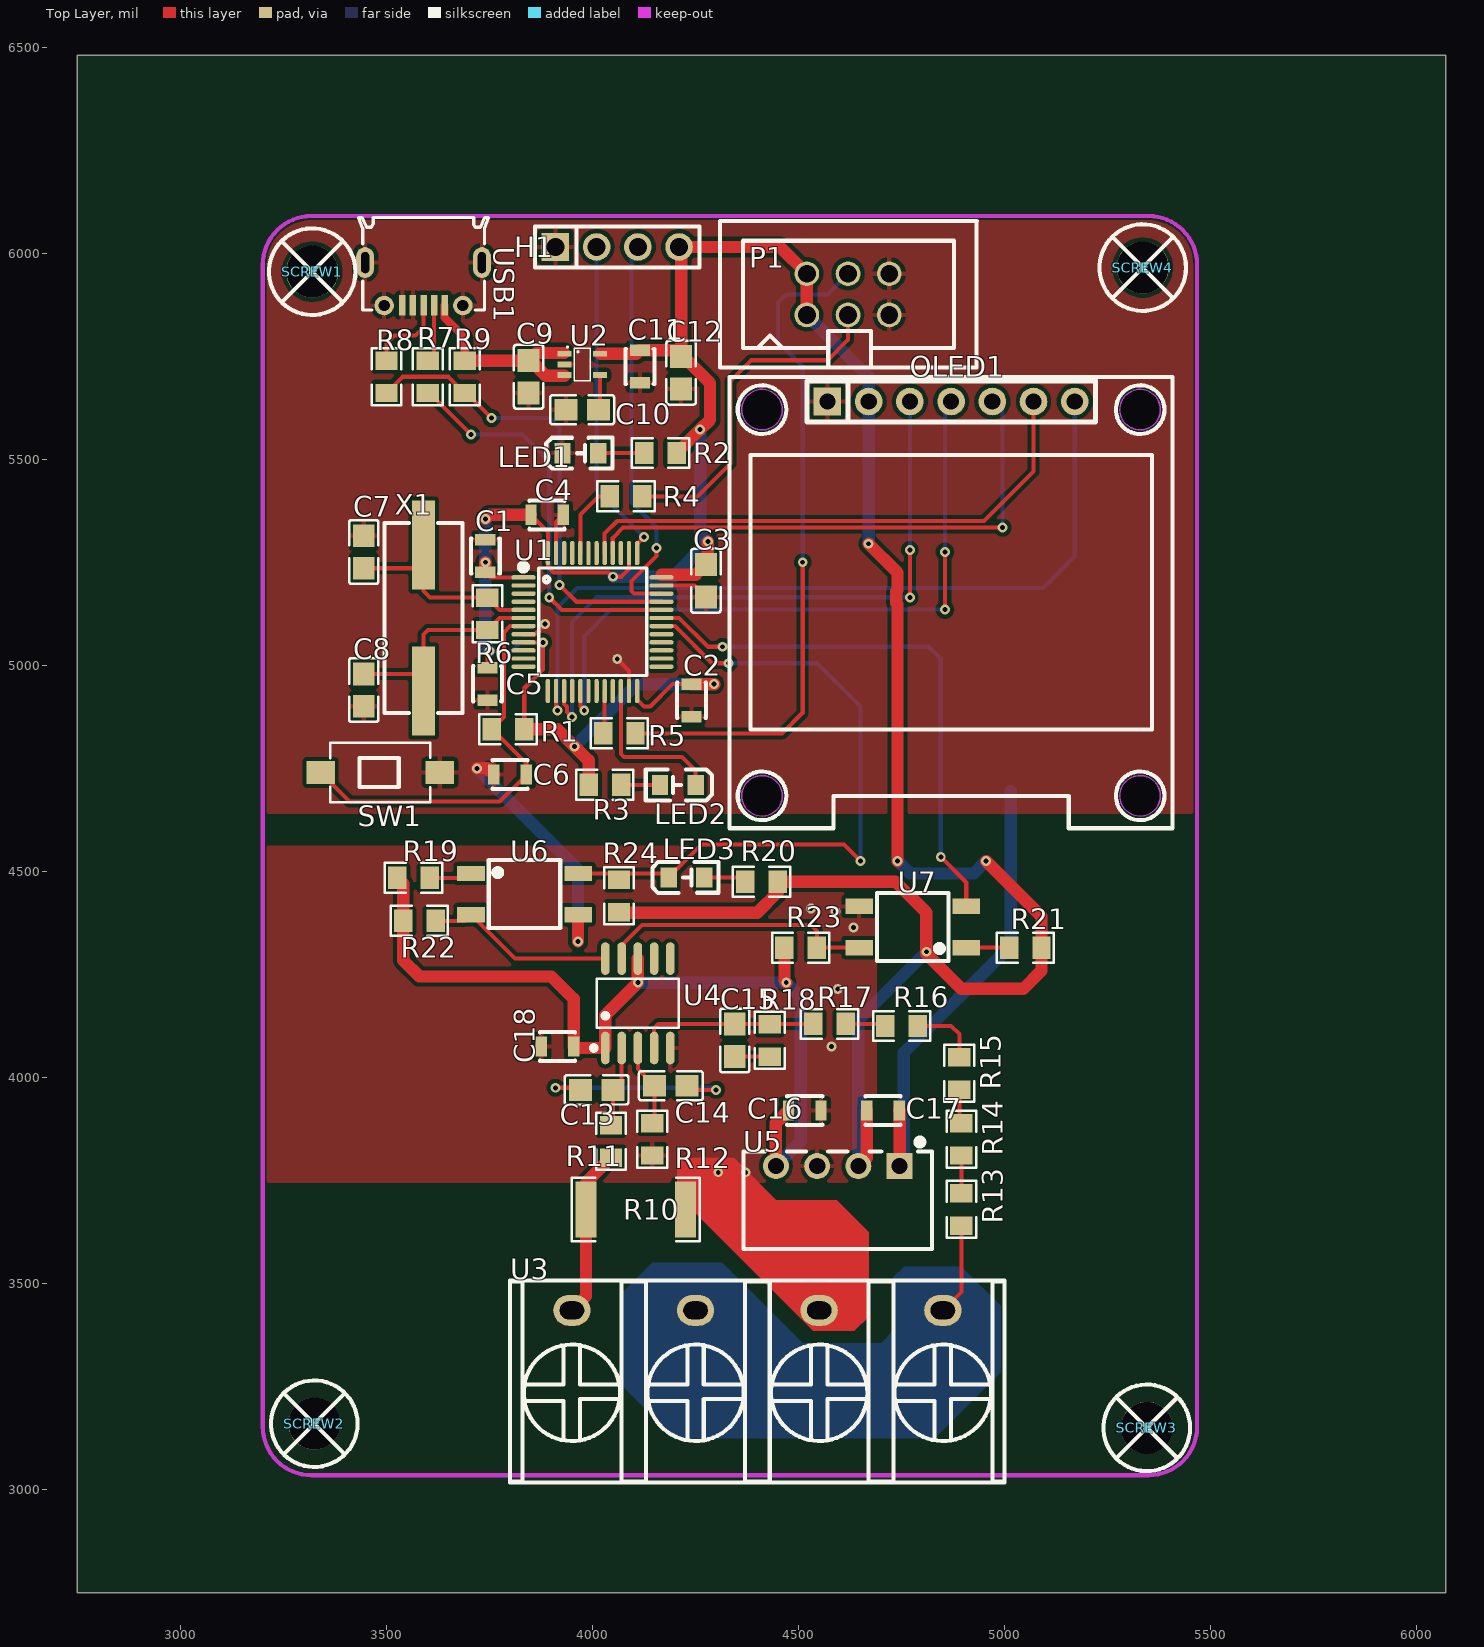
[diagram p0: Top Layer view]
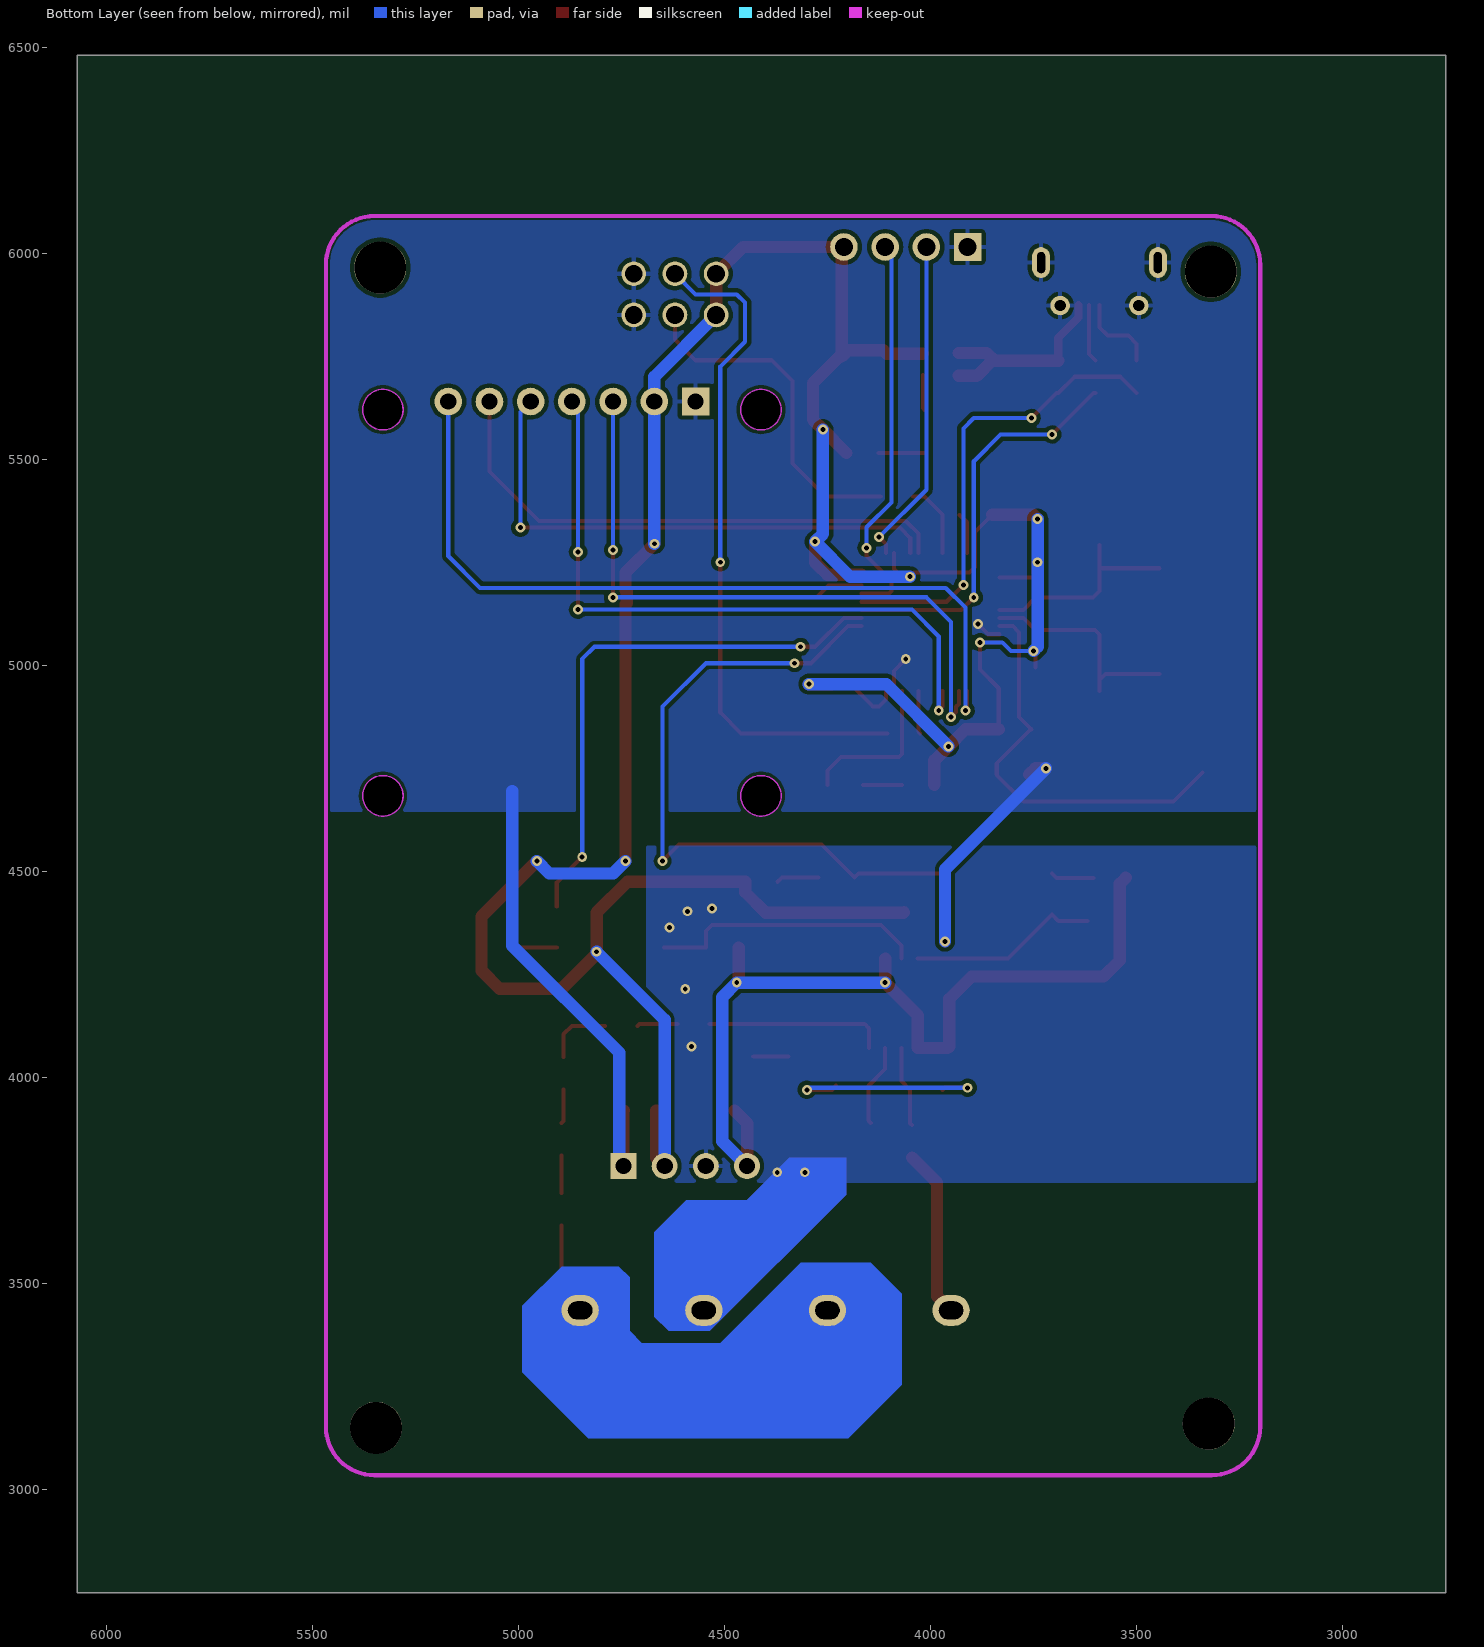
[diagram p1: Bottom Layer view, seen from below]
# Altium PCB MISC61948.pcbdoc
Units mil, origin at the board's own origin, x right, y up, seen from the top; angles counter-clockwise.
Board outline 3320 x 3730 mil, 2 copper layers (Top Layer, Bottom Layer), stack 62.206 mil thick; 62 components, 45 nets, 203 pads, 47 vias.

## Layer stack, top to bottom
Top Solder Mask Layer: solder mask 0.394, Dk 3.3
Top Layer: signal copper 1.379
Dielectric1: surface 59.449, FR4, Dk 4.5
Bottom Layer: signal copper 1.378
Bottom Solder Mask Layer: solder mask 0.394, Dk 3.3

## Board outline
6070,2750 2750,2750 2750,6480 6070,6480

## Design rules (kind name [scope] priority, off if disabled: settings)
BoardOutlineClearance safeClearance_1 [All] p2: genericclearance=6 ignorepadtopadclearanceinfootprint=FALSE except(0: Arc-SplitContinuation Track-SplitContinuation SMDPad-SplitContinuation THPad-SplitContinuation Via-SplitContinuation Fill-SplitContinuation Region-SplitContinuation Poly-SplitContinuation Text-SplitContinuation Hole-SplitContinuation; 6: Arc-CutoutEdge Track-CutoutEdge SMDPad-CutoutEdge THPad-CutoutEdge Via-CutoutEdge Fill-CutoutEdge Region-CutoutEdge Text-CutoutEdge Hole-CutoutEdge; 10: Poly-OutlineEdge Poly-CutoutEdge; 11.8: Arc-OutlineEdge Track-OutlineEdge SMDPad-OutlineEdge THPad-OutlineEdge Via-OutlineEdge Fill-OutlineEdge Region-OutlineEdge Text-OutlineEdge Hole-OutlineEdge)
Clearance safeClearance [All] p1: gap=6 ignorepadtopadclearanceinfootprint=FALSE except(10: Poly-Track Poly-SMDPad Poly-THPad Poly-Via Poly-Fill Poly-Region Poly-Poly Poly-Arc Poly-Text Poly-Hole)
DiffPairsRouting differentialPair [All] p1: maxlimit=6 minlimit=6 mostfreqgap=6 toplayer_minwidth=5 toplayer_prefwidth=10 toplayer_maxwidth=100 toplayer_mingap=6 toplayer_prefgap=6 toplayer_maxgap=6 bottomlayer_minwidth=5 bottomlayer_prefwidth=10 bottomlayer_maxwidth=100 bottomlayer_mingap=6 bottomlayer_prefgap=6 bottomlayer_maxgap=6 maxuncoupledlength=10
HoleToHoleClearance otherClearance [All] p1: gap=11.2 allowstackedmicrovias=TRUE
Length netLength [All] p1: minlimit=0 maxlimit=0
MatchedLengths netLengthTolerance [All] p1: tolerance=1000
PasteMaskExpansion pasteMaskExpansion [All] p1: expansion=0
PlaneConnect innerPlane [All] p1: planeconnectstyle=Relief reliefexpansion=20 reliefentries=4 reliefconductorwidth=10 reliefairgap=10
PolygonConnect copperRegion [(InNet('GND') OR InNet('AGND'))] p1: connectstyle=Relief reliefconductorwidth=10 reliefentries=4 polygonreliefangle="90 Angle" airgapwidth=10 via.connectstyle=Relief via.reliefconductorwidth=10 via.reliefentries=4 via.polygonreliefangle="90 Angle" via.airgapwidth=10
RoutingVias viaSize [All] p1: holewidth=12 width=24 viastyle="Through Hole" minholewidth=11.8 minwidth=19.7 maxholewidth=236.2 maxwidth=393.7
SolderMaskExpansion solderMaskExpansion [IsVia] p1: expansion=-1000 istentingtop=TRUE
SolderMaskExpansion solderMaskExpansion [All] p2: expansion=2 istentingtop=FALSE
Width power [(InNet('GND') OR InNet('VCC3.3') OR InNet('+5V') OR InNet('AGND') OR InNet('VCC'))] p1: maxlimit=10 minlimit=10 preferedwidth=10 toplayer_minwidth=10 toplayer_maxwidth=100 toplayer_prefwidth=30 bottomlayer_minwidth=10 bottomlayer_maxwidth=100 bottomlayer_prefwidth=30
Width trackWidth [All] p2: maxlimit=10 minlimit=10 preferedwidth=10 toplayer_minwidth=5 toplayer_maxwidth=100 toplayer_prefwidth=10 bottomlayer_minwidth=5 bottomlayer_maxwidth=100 bottomlayer_prefwidth=10

## Components (designator, comment, footprint, x,y, rotation, side; value= is the part's Value field where it differs from the comment)
C1 "100nF" CAP-SMD_L2.0-W1.25 3740,5265 r270 top
C2 "100nF" CAP-SMD_L2.0-W1.25 4240,4915 r90 top
C3 "2.2uF" C0805 4275,5205 r270 top
C4 "100nF" CAP-SMD_L2.0-W1.25 3890,5365 r180 top
C5 "100nF" CAP-SMD_L2.0-W1.25 3745,4955 r90 top
C6 "100nF" CAP-SMD_L2.0-W1.25 3800,4735 r180 top
C7 "22pF" C0805 3445,5275 r90 top
C8 "22pF" C0805 3445,4940 r270 top
C9 "1uF" C0805 3845,5700 r90 top
C10 "22nF" C0805 3975,5620 r0 top
C11 "100nF" CAP-SMD_L2.0-W1.25 4115,5725 r270 top
C12 "10uF" C0805 4215,5710 r90 top
C13 "68nF" C0805 4010,3970 r180 top
C14 "68nF" C0805 4190,3980 r180 top
C15 "68nF" C0805 4345,4090 r270 top
C16 "100nF" CAP-SMD_L2.0-W1.25 4515,3920 r180 top
C17 "100nF" CAP-SMD_L2.0-W1.25 4705,3920 r180 top
C18 "100nF" CAP-SMD_L2.0-W1.25 3915,4075 r180 top
H1 "PZ254V-11-04P" HDR-TH_4P-P2.54-V-M 4060,6015 r0 top
LED1 "" LED_0805 3972.31,5514.53 r0 top
LED2 "" LED_0805 4205,4710 r180 top
LED3 "" LED_0805 4230,4485 r0 top
OLED1 "HS96L01W4S03" OLED-TH_HS96L01W4S03 4870,5640 r0 top
P1 "2.54-2*3P pin header" IDC-TH_6P-P2.54_C11214 4620,5900 r0 top
R1 "10kΩ" R0805 3795,4845 r0 top
R2 "1kΩ" R0805 4165,5515 r0 top
R3 "1kΩ" R0805 4030,4710 r180 top
R4 "10kΩ" R0805 4081.26,5410 r180 top
R5 "10kΩ" R0805 4065,4835 r0 top
R6 "1MΩ" R0805 3745,5125 r90 top
R7 "20Ω" R0805 3600,5700 r270 top
R8 "20Ω" R0805 3500,5700 r270 top
R9 "4.7kΩ" R0805 3690,5700 r270 top
R10 "3mΩ" R2512 4105,3680 r180 top
R11 "510Ω" R0805 4045,3845 r270 top
R12 "510Ω" R0805 4145,3850 r270 top
R13 "390kΩ" R0805 4895,3680 r270 top
R14 "390kΩ" R0805 4895,3850 r270 top
R15 "390kΩ" R0805 4890,4010 r270 top
R16 "390kΩ" R0805 4750,4125 r0 top
R17 "390kΩ" R0805 4575,4130 r0 top
R18 "510Ω" R0805 4430,4090 r270 top
R19 "1kΩ" R0805 3565.63,4484.37 r180 top
R20 "1kΩ" R0805 4410,4475 r180 top
R21 "1kΩ" R0805 5050,4315 r0 top
R22 "10kΩ" R0805 3580,4380 r180 top
R23 "10kΩ" R0805 4505,4315 r180 top
R24 "3.3kΩ" R0805 4064.37,4440.63 r90 top
SCREW1 "" M3螺丝 3320,5955 r0 top
SCREW2 "" M3螺丝 3325,3160 r0 top
SCREW3 "" M3螺丝 5345,3150 r0 top
SCREW4 "" M3螺丝 5335,5965 r0 top
SW1 "TS1305-TZ43HBM" SW-SMD_L6.0-W3.5-LS8.0_TS04-TBW1FH4.3 3485,4740 r180 top
U1 "STM32F103C8T6" LQFP-48_L7.0-W7.0-P0.50-LS9.0-BL 4000,5105 r270 top
U2 "RT9193-33GU5" SC-70-5_L2.0-W1.3-P0.65-LS2.1-BL 3975,5730 r270 top
U3 "DBT10-7.62-4P-GN-P" CONN-TH_DBT10-7.62-4P 4400,3435 r0 top
U4 "BL0942" SSOP-10_L4.9-W3.9-P1.00-LS6.0-BL 4110,4180 r0 top
U5 "B0303S-1W" PWRM-TH_BXXXXS-1W 4595,3785 r180 top
U6 "EL357N(C)(TA)-G" OPTO-SMD-4_L4.4-W4.1-P2.54-LS7.0-TL 3835,4445 r0 top
U7 "EL357N(C)(TA)-G" OPTO-SMD-4_L4.4-W4.1-P2.54-LS7.0-TL 4776.77,4365 r180 top
USB1 "920-E52A2021S10100" MICRO-USB-SMD_5P-P0.65-H-F_C10418 3590,5925 r180 top
X1 "8MHz" CRYSTAL-SMD_L11.4-W4.7-LS12.7 3590,5115 r90 top

## Footprints (in the part's own frame and the unit in brackets; to place one, negate y for a bottom-side part, rotate by r counter-clockwise, add the part's x,y. Pads: shape width x height; smd on the part's side, far side on the other; paste and mask are expansions set on the pad)
C0805 [mm]
  rect 1.41x1.35 smd paste-100 mask+0.051: 1(-1,0) 2(1,0)
  silkscreen extent -1.96,-0.9 1.96,0.9
CAP-SMD_L2.0-W1.25 [mm]
  rect 0.7x1.25 smd: 1(-1,0) 2(1,0)
  silkscreen extent -1.08,-0.89 1.08,0.89
CONN-TH_DBT10-7.62-4P [mm]
  oval 2.3x1.9 hole 1.1 slot 1.5 at 0 deg: 1(-11.43,0) 2(-3.81,0) 3(3.81,0) 4(11.43,0)
  silkscreen extent -15.24,-10.6 15.24,1.85
CRYSTAL-SMD_L11.4-W4.7-LS12.7 [mm]
  rect 5.5x1.4 smd: 1(-4.5,0) 2(4.5,0)
  silkscreen extent -5.85,-2.4 5.85,2.4
HDR-TH_4P-P2.54-V-M [mm]
  rect 1.7x1.7 hole 1.1: 1(-3.81,0)
  round 1.7 hole 1.1: 2(-1.27,0) 3(1.27,0) 4(3.81,0)
  silkscreen extent -5.08,-1.27 5.08,1.27
IDC-TH_6P-P2.54_C11214 [mil]
  round 60 hole 43.3: 1(-100,-50) 2(-100,50) 3(0,-50) 4(0,50) 5(100,-50) 6(100,50)
  silkscreen extent -311,-177 312,178
LED_0805 [mm]
  rect 1x1.25 smd paste+0 mask+0.051: 1(-1.15,0.005) 2(1.05,0.005)
  silkscreen extent -2.15,-0.94 1.93,0.97
LQFP-48_L7.0-W7.0-P0.50-LS9.0-BL [mm]
  oval 0.27x1.5 smd paste+0 mask+0.05: 1(-2.75,-4.25) 2(-2.25,-4.25) 3(-1.75,-4.25) 4(-1.25,-4.25) 5(-0.75,-4.25) 6(-0.25,-4.25) 7(0.25,-4.25) 8(0.75,-4.25) 9(1.25,-4.25) 10(1.75,-4.25) 11(2.25,-4.25) 12(2.75,-4.25) 25(2.75,4.25) 26(2.25,4.25) 27(1.75,4.25) 28(1.25,4.25) 29(0.75,4.25) 30(0.25,4.25) 31(-0.25,4.25) 32(-0.75,4.25) 33(-1.25,4.25) 34(-1.75,4.25) 35(-2.25,4.25) 36(-2.75,4.25)
  oval 1.5x0.27 smd paste+0 mask+0.05: 13(4.25,-2.75) 14(4.25,-2.25) 15(4.25,-1.75) 16(4.25,-1.25) 17(4.25,-0.75) 18(4.25,-0.25) 19(4.25,0.25) 20(4.25,0.75) 21(4.25,1.25) 22(4.25,1.75) 23(4.25,2.25) 24(4.25,2.75) 37(-4.25,2.75) 38(-4.25,2.25) 39(-4.25,1.75) 40(-4.25,1.25) 41(-4.25,0.75) 42(-4.25,0.25) 43(-4.25,-0.25) 44(-4.25,-0.75) 45(-4.25,-1.25) 46(-4.25,-1.75) 47(-4.25,-2.25) 48(-4.25,-2.75)
  silkscreen extent -3.59,-4.46 3.3,3.34
M3螺丝 [mil]
  round 126 hole 126 paste+0 mask+4: 1(0,0)
  silkscreen extent -105,-105 105,105
MICRO-USB-SMD_5P-P0.65-H-F_C10418 [mm]
  rect 0.4x1.25 smd paste-100 mask+0.05: 1(-1.3,1.3) 2(-0.65,1.3) 3(0,1.3) 4(0.65,1.3) 5(1.3,1.3)
  round 1.2 hole 0.7 paste+0 mask+0.05: SH0(-2.425,1.325) SH3(2.425,1.325)
  oval 1.1x1.9 hole 0.5 slot 1.3 at 90 deg: SH1(-3.6,-1.325) SH2(3.6,-1.325)
  silkscreen extent -4,-4.1 4,1.6
OLED-TH_HS96L01W4S03 [mm]
  rect 1.7x1.7 hole 1: 1(-7.62,0)
  round 1.7 hole 1: 2(-5.08,0) 3(-2.54,0) 4(0,0) 5(2.54,0) 6(5.08,0) 7(7.62,0)
  Board Outline Layer circle w0.003: c11.65,-0.5 r1.25
  Board Outline Layer circle w0.003: c-11.65,-0.5 r1.25
  Board Outline Layer circle w0.003: c-11.65,-24.3 r1.25
  Board Outline Layer circle w0.003: c11.65,-24.3 r1.25
  Board Outline Layer region: 12.9,-0.5 12.776,-1.042 12.429,-1.477 11.928,-1.719 11.372,-1.719 10.871,-1.477 10.524,-1.042 10.4,-0.5 10.4,-0.5 10.524,0.042 10.871,0.477 11.372,0.719 11.928,0.719 12.429,0.477 12.776,0.042 12.9,-0.5
  Board Outline Layer region: 12.9,-0.5 12.89,-0.657 12.861,-0.811 12.812,-0.96 12.745,-1.102 12.661,-1.235 12.561,-1.356 12.447,-1.463 12.32,-1.555 12.182,-1.631 12.036,-1.689 11.884,-1.728 11.728,-1.747 11.571,-1.747 11.416,-1.728 11.264,-1.689 11.118,-1.631 10.98,-1.555 10.853,-1.463 10.739,-1.356 10.639,-1.235 10.555,-1.102 10.488,-0.96 10.439,-0.811 10.41,-0.657 10.4,-0.5 10.41,-0.343 10.439,-0.189 10.488,-0.04 10.555,0.102 10.639,0.235 10.739,0.356 10.853,0.463 10.98,0.556 11.118,0.631 11.264,0.689 11.416,0.728 11.571,0.748 11.728,0.748 11.884,0.728 12.036,0.689 12.182,0.631 12.32,0.556 12.447,0.463 12.561,0.356 12.661,0.235 12.745,0.102 12.812,-0.04 12.861,-0.189 12.89,-0.343
  Board Outline Layer region: -10.4,-0.5 -10.524,-1.042 -10.871,-1.477 -11.372,-1.719 -11.928,-1.719 -12.429,-1.477 -12.776,-1.042 -12.9,-0.5 -12.9,-0.5 -12.776,0.042 -12.429,0.477 -11.928,0.719 -11.372,0.719 -10.871,0.477 -10.524,0.042 -10.4,-0.5
  Board Outline Layer region: -10.4,-0.5 -10.41,-0.657 -10.439,-0.811 -10.488,-0.96 -10.555,-1.102 -10.639,-1.235 -10.739,-1.356 -10.853,-1.463 -10.98,-1.555 -11.118,-1.631 -11.264,-1.689 -11.416,-1.728 -11.571,-1.747 -11.728,-1.747 -11.884,-1.728 -12.036,-1.689 -12.182,-1.631 -12.32,-1.555 -12.447,-1.463 -12.561,-1.356 -12.661,-1.235 -12.745,-1.102 -12.812,-0.96 -12.861,-0.811 -12.89,-0.657 -12.9,-0.5 -12.89,-0.343 -12.861,-0.189 -12.812,-0.04 -12.745,0.102 -12.661,0.235 -12.561,0.356 -12.447,0.463 -12.32,0.556 -12.182,0.631 -12.036,0.689 -11.884,0.728 -11.728,0.748 -11.571,0.748 -11.416,0.728 -11.264,0.689 -11.118,0.631 -10.98,0.556 -10.853,0.463 -10.739,0.356 -10.639,0.235 -10.555,0.102 -10.488,-0.04 -10.439,-0.189 -10.41,-0.343
  Board Outline Layer region: -10.4,-24.3 -10.524,-24.842 -10.871,-25.277 -11.372,-25.519 -11.928,-25.519 -12.429,-25.277 -12.776,-24.842 -12.9,-24.3 -12.9,-24.3 -12.776,-23.758 -12.429,-23.323 -11.928,-23.081 -11.372,-23.081 -10.871,-23.323 -10.524,-23.758 -10.4,-24.3
  Board Outline Layer region: -10.4,-24.3 -10.41,-24.457 -10.439,-24.611 -10.488,-24.76 -10.555,-24.902 -10.639,-25.035 -10.739,-25.156 -10.853,-25.263 -10.98,-25.355 -11.118,-25.431 -11.264,-25.489 -11.416,-25.528 -11.571,-25.547 -11.728,-25.547 -11.884,-25.528 -12.036,-25.489 -12.182,-25.431 -12.32,-25.355 -12.447,-25.263 -12.561,-25.156 -12.661,-25.035 -12.745,-24.902 -12.812,-24.76 -12.861,-24.611 -12.89,-24.457 -12.9,-24.3 -12.89,-24.143 -12.861,-23.989 -12.812,-23.84 -12.745,-23.698 -12.661,-23.565 -12.561,-23.444 -12.447,-23.337 -12.32,-23.245 -12.182,-23.169 -12.036,-23.111 -11.884,-23.072 -11.728,-23.052 -11.571,-23.052 -11.416,-23.072 -11.264,-23.111 -11.118,-23.169 -10.98,-23.245 -10.853,-23.337 -10.739,-23.444 -10.639,-23.565 -10.555,-23.698 -10.488,-23.84 -10.439,-23.989 -10.41,-24.143
  Board Outline Layer region: 12.9,-24.3 12.776,-24.842 12.429,-25.277 11.928,-25.519 11.372,-25.519 10.871,-25.277 10.524,-24.842 10.4,-24.3 10.4,-24.3 10.524,-23.758 10.871,-23.323 11.372,-23.081 11.928,-23.081 12.429,-23.323 12.776,-23.758 12.9,-24.3
  Board Outline Layer region: 12.9,-24.3 12.89,-24.457 12.861,-24.611 12.812,-24.76 12.745,-24.902 12.661,-25.035 12.561,-25.156 12.447,-25.263 12.32,-25.355 12.182,-25.431 12.036,-25.489 11.884,-25.528 11.728,-25.547 11.571,-25.547 11.416,-25.528 11.264,-25.489 11.118,-25.431 10.98,-25.355 10.853,-25.263 10.739,-25.156 10.639,-25.035 10.555,-24.902 10.488,-24.76 10.439,-24.611 10.41,-24.457 10.4,-24.3 10.41,-24.143 10.439,-23.989 10.488,-23.84 10.555,-23.698 10.639,-23.565 10.739,-23.444 10.853,-23.337 10.98,-23.245 11.118,-23.169 11.264,-23.111 11.416,-23.072 11.571,-23.052 11.728,-23.052 11.884,-23.072 12.036,-23.111 12.182,-23.169 12.32,-23.245 12.447,-23.337 12.561,-23.444 12.661,-23.565 12.745,-23.698 12.812,-23.84 12.861,-23.989 12.89,-24.143
  Multi-Layer board cut-out: 12.9,-0.5 12.776,-1.042 12.429,-1.477 11.928,-1.719 11.372,-1.719 10.871,-1.477 10.524,-1.042 10.4,-0.5 10.4,-0.5 10.524,0.042 10.871,0.477 11.372,0.719 11.928,0.719 12.429,0.477 12.776,0.042 12.9,-0.5
  Multi-Layer board cut-out: -10.4,-0.5 -10.524,-1.042 -10.871,-1.477 -11.372,-1.719 -11.928,-1.719 -12.429,-1.477 -12.776,-1.042 -12.9,-0.5 -12.9,-0.5 -12.776,0.042 -12.429,0.477 -11.928,0.719 -11.372,0.719 -10.871,0.477 -10.524,0.042 -10.4,-0.5
  Multi-Layer board cut-out: -10.4,-24.3 -10.524,-24.842 -10.871,-25.277 -11.372,-25.519 -11.928,-25.519 -12.429,-25.277 -12.776,-24.842 -12.9,-24.3 -12.9,-24.3 -12.776,-23.758 -12.429,-23.323 -11.928,-23.081 -11.372,-23.081 -10.871,-23.323 -10.524,-23.758 -10.4,-24.3
  Multi-Layer board cut-out: 12.9,-24.3 12.776,-24.842 12.429,-25.277 11.928,-25.519 11.372,-25.519 10.871,-25.277 10.524,-24.842 10.4,-24.3 10.4,-24.3 10.524,-23.758 10.871,-23.323 11.372,-23.081 11.928,-23.081 12.429,-23.323 12.776,-23.758 12.9,-24.3
  silkscreen extent -13.65,-26.3 13.65,1.5
OPTO-SMD-4_L4.4-W4.1-P2.54-LS7.0-TL [mm]
  rect 1.7x0.95 smd: 1(-3.3,1.27) 2(-3.3,-1.27) 3(3.3,-1.27) 4(3.3,1.27)
  silkscreen extent -2.2,-2.1 2.2,2.1
PWRM-TH_BXXXXS-1W [mm]
  rect 1.6x1.6 hole 1: 1(-3.81,0)
  round 1.6 hole 1: 2(-1.27,0) 3(1.27,0) 4(3.81,0)
  silkscreen extent -5.8,-1.68 5.8,5.1
R0805 [mm]
  rect 1.133x1.377 smd paste-100 mask+0.051: 1(-1,0) 2(1,0)
  silkscreen extent -1.76,-0.92 1.76,0.92
R2512 [mil]
  rect 50.49x136.06 smd paste-3937.01 mask+2: 1(-120.72,0) 2(120.72,0)
  silkscreen extent -155,-77 155,77
SC-70-5_L2.0-W1.3-P0.65-LS2.1-BL [mm]
  rect 0.35x0.85 smd paste+0 mask+0.05: 1(-0.65,-1.1) 2(0,-1.1) 3(0.65,-1.1) 4(0.65,1.1) 5(-0.65,1.1)
  silkscreen extent -1.12,-0.96 1,0.5
SSOP-10_L4.9-W3.9-P1.00-LS6.0-BL [mm]
  oval 0.525x2.014 smd: 1(-2,-2.757) 2(-1,-2.757) 3(0,-2.757) 4(1,-2.757) 5(2,-2.757) 6(2,2.757) 7(1,2.757) 8(0,2.757) 9(-1,2.757) 10(-2,2.757)
  silkscreen extent -2.86,-2.91 2.53,1.52
SW-SMD_L6.0-W3.5-LS8.0_TS04-TBW1FH4.3 [mm]
  rect 1.74x1.4 smd: 1(-3.67,0) 2(3.67,0)
  silkscreen extent -3.08,-1.83 3.08,1.83

## Via types
v1: diameter 24, hole 12, Top Layer to Bottom Layer, 47 vias

## Nets (pads, with @x,y where several pads share a name; then routed paths per layer and width w, separated by ;. In a path a pad name is that pad's centre, name@x,y a point inside that pad or via, vN(x,y) a via of type N, cw(c..) or ccw(c..) an arc to the next point about the centre after c; other vN are vias at no path point)
$1N32: R7.1 USB1.2 | length 140.9
  Top Layer w10: R7.1 3615.59,5754.96 USB1.2
$1N33: R8.1 USB1.3 | length 201
  Top Layer w10: R8.1 3500,5780 3520,5800 3570,5800 3590,5820 USB1.3
$1N43: C10.2 U2.4 | length 86
  Top Layer w10: C10.2 4018.3,5623.94 U2.4
$1N56: P1.3 R4.1 | length 833.9
  Top Layer w10: R4.1 4255,5410 4335,5490 4335,5690 4385,5740 4570,5740 4620,5790 P1.3
$1N60: P1.4 R5.2 | length 1645.2
  Top Layer w10: R5.2 4460,4835 4510,4885 v1(4510,5250)
  Bottom Layer w10: v1(4510,5250) 4510,5725 4450,5785 4450,5880 4470,5900 4570,5900 P1.4
$1N68: LED2.2 R3.1 | length 94.4
  Top Layer w10: R3.1 4069.57,4709.8 LED2.2
$1N69: LED1.2 R2.1 | length 112.1
  Top Layer w10: LED1.2 4013.92,5515 R2.1
$1N90: C13.2 C14.1 | length 529.5
  Top Layer w10: v1(3910,3975) 3965.63,3975 C13.2 ; C14.1 4239.37,3970 v1(4300,3970)
  Bottom Layer w10: v1(3910,3975) 4295,3975 v1(4300,3970)
$1N91: C13.1 R11.1 U4.2 | length 197.7
  Top Layer w10: R11.1 4049.37,3888.74 C13.1 4070.63,3991.26 U4.2
$1N92: C14.2 R12.1 U4.3 | length 201.3
  Top Layer w10: U4.3 4110,4020.63 C14.2 4150.63,3895 R12.1
$1N94: C15.1 R17.1 R18.1 U4.4 | length 438.6
  Top Layer w10: U4.4 4149.37,4119.37 4159.37,4129.37 C15.1 R18.1 4535,4129.37 R17.1
$1N98: R13.1 R14.2 | length 91.3
  Top Layer w10: R13.1 R14.2
$1N99: R14.1 R15.2 | length 83.3
  Top Layer w10: R15.2 4890,3894.37 R14.1
$1N100: R15.1 R16.2 | length 164.5
  Top Layer w10: R16.2 4870,4125 4890,4105 R15.1
$1N101: R16.1 R17.2 | length 98.3
  Top Layer w10: R17.2 4705.63,4130 R16.1
$1N102: C15.2 R18.2 | length 85
  Top Layer w10: C15.2 R18.2
$1N108: LED3.2 R20.2 | length 103.5
  Top Layer w10: LED3.2 4360.43,4485.2 R20.2
$1N110: R19.1 U6.1 | length 104.5
  Top Layer w10: R19.1 3694.45,4484.37 U6.1
$1N112: R21.1 U7.1 | length 103.9
  Top Layer w10: U7.1 R21.1
+5V: C9.2 R9.1 U2.1 U2.3 USB1.1 | length 506.2
  Top Layer w20: USB1.1 3641.18,5843.82 3690,5795 R9.1
  Top Layer w30: R9.1 C9.2 ; U2.3@3931.7,5702.11 3887.55,5702.11 3850.29,5739.37 C9.2 ; U2.1@3931.7,5757.89 3863.52,5757.89 C9.2
AGND: C16.1 C18.2 R10.1 R12.2 U3.3 U4.5 U5.3 U7.3
  other v1: 4305,3770 4371.77,3770 4580,4075 4595,4215 4633.39,4363.51 4589.67,4403.21 4530,4410
B00T1: R5.1 U1.20 | length 104.3
  Top Layer w10: R5.1 4029.53,4838.9 U1.20
BOOT0: R4.2 U1.44 | length 183
  Top Layer w10: U1.44 3970.47,5365.47 4015,5410 R4.2
CS: OLED1.7 U1.14 | length 1980.9
  Top Layer w10: U1.14 3911.42,4893.58 v1(3915,4890)
  Bottom Layer w10: v1(3915,4890) 3915,5140 3963,5188 5093,5188 5170,5265 OLED1.7
DC: OLED1.6 U1.41 | length 1320
  Top Layer w10: U1.41 4029.53,5319.53 4060,5350 4950,5350 5070,5470 OLED1.6
GND: C1.1 C2.1 C3.2 C4.1 C5.1 C6.2 C7.2 C8.2 C9.1 C10.1 C11.2 C12.1 C17.1 H1.1 LED1.1 OLED1.1 P1.5 P1.6 SW1.1 U1.8 U1.23 U1.35 U1.47 U2.2 U5.1 U6.3 USB1.4 USB1.5 USB1.SH0 USB1.SH1 USB1.SH2 USB1.SH3 | length 2122.3
  Top Layer w10: U1.8 3860.47,5075.47 v1(3885,5100) ; U1.47 3911.42,5347.05 C4.1 ; v1(4060,5015) 4088.58,4986.42 U1.23 ; U1.35 4247.05,5193.58 C3.2
  Top Layer w30: v1(3720,4750) 3745.63,4750 C6.2 ; v1(3964.92,4330) U6.3 ; C17.1 4745,3919.37 U5.1
  Bottom Layer w30: v1(3720,4750) 3964.92,4505.08 v1(3964.92,4330) ; 4755,3820 4755,4060 5015,4320 5015,4695
INL: R13.2 U3.2 U3.4 | length 224.3
  Top Layer w10: U3.4 4895,3480 R13.2
LED: LED2.1 U1.22 | length 385.7
  Top Layer w10: U1.22 4068.9,4785 4075.97,4777.93 4217.07,4777.93 4250.28,4744.72 LED2.1
NRST: C6.1 R1.1 SW1.2 U1.7 | length 1001
  Top Layer w10: SW1.2 3410.51,4670 3775,4670 3839.37,4734.37 C6.1 3839.37,4761.26 R1.1 3785,4874.37 3785,5080 3800.16,5095.16 U1.7
ORX: U1.31 U7.2 | length 1344.6
  Top Layer w10: U1.31 4210.16,5114.84 4280,5045 v1(4315,5045) ; v1(4845,4535) 4906.69,4473.31 U7.2
  Bottom Layer w10: v1(4315,5045) 4815,5045 4845,5015 v1(4845,4535)
OSCI: C7.1 R6.2 U1.5 X1.2 | length 518.7
  Top Layer w10: C7.1 X1.2@3590,5235.63 ; X1.2 X1.2@3590,5235.63 ; U1.5 3774.84,5134.53 R6.2 3605.63,5164.37 3590,5180 X1.2@3590,5235.63
OSCO: C8.1 R6.1 U1.6 X1.1 | length 547.3
  Top Layer w10: C8.1 3575.63,4979.37 X1.1@3590,4965 ; X1.1 X1.1@3590,4965 ; U1.6 3774.21,5114.84 R6.1 3600.63,5085.63 3590,5075 X1.1@3590,4965
OTX: LED3.1 R24.2 U1.30 U6.4 | length 1677.3
  Top Layer w10: U6.4 4174.92,4495 LED3.1 4264.52,4565 4610,4565 v1(4650,4525) ; U1.30 4199.84,5095.16 4290,5005 v1(4330,5005)
  Bottom Layer w10: v1(4330,5005) 4545,5005 4650,4900 v1(4650,4525)
OUT_N: R10.2 R11.2 U3.1 | length 410
  Top Layer w30: U3.1 3984.28,3469.28 R10.2 3984.28,3744.91 R11.2
PA11: R7.2 U1.32 | length 978.5
  Top Layer w10: R7.2 3604.37,5660.63 v1(3705,5560) ; v1(3895,5165) 3925.47,5134.53 U1.32
  Bottom Layer w10: v1(3705,5560) 3830,5560 3895,5495 v1(3895,5165)
PA12: R8.2 R9.2 U1.33 | length 1132.3
  Top Layer w10: R8.2 3539.37,5700 3650.63,5700 R9.2 3694.37,5660.63 v1(3755,5600) ; v1(3920,5195) 3960.79,5154.21 U1.33
  Bottom Layer w10: v1(3755,5600) 3895,5600 3920,5575 v1(3920,5195)
RES: OLED1.5 U1.40 | length 1309.3
  Top Layer w10: U1.40 4049.21,5309.21 4074,5334 v1(4995,5334)
  Bottom Layer w10: OLED1.5 4995,5615 v1(4995,5334)
RX: R23.1 U4.9 U7.4 | length 675.4
  Top Layer w10: U4.9 4070.63,4320.63 4120,4370 4530,4370 4544.37,4355.63 R23.1 U7.4
SCL: OLED1.3 U1.15 | length 1620.4
  Top Layer w10: U1.15 3931.1,4906.43 3938,4899.53 3938,4887 v1(3950,4875) ; v1(4770,5165) v1(4770,5280)
  Bottom Layer w10: v1(3950,4875) 3950,5105 4010,5165 v1(4770,5165) ; v1(4770,5280) OLED1.3
SDA: OLED1.4 U1.17 | length 1644.8
  Top Layer w10: U1.17 3970.47,4899.53 v1(3980,4890) ; v1(4855,5135) v1(4855,5275)
  Bottom Layer w10: v1(3980,4890) 3980,5070 4045,5135 v1(4855,5135) ; v1(4855,5275) 4855,5625 OLED1.4
SWCLK: H1.2 U1.37 | length 797.2
  Top Layer w10: U1.37 4108.27,5294.27 v1(4125,5311)
  Bottom Layer w10: H1.2 4010,5426 v1(4125,5311)
SWDIO: H1.3 U1.34 | length 965.8
  Top Layer w10: v1(4155,5285) 4155,5265 4095,5205 4095,5180 4101.1,5173.9 U1.34
  Bottom Layer w10: H1.3 4095,6000 4095,5395 4155,5335 v1(4155,5285)
TX: R22.1 U4.10 U6.2 | length 462.2
  Top Layer w10: R22.1 3690.08,4380 U6.2 3811.55,4288.53 U4.10
VCC: C16.2 C18.1 R19.2 R22.2 R23.2 U4.1 U4.8 U5.4 | length 2181
  Top Layer w30: R19.2 3540.63,4470 R22.2 3540.63,4284.37 3580,4245 3900,4245 3954.37,4190.63 C18.1 3957.9,4071.47 U4.1 4031.26,4151.26 v1(4110,4230) U4.8 ; U5.4 4445,3889.37 C16.2 ; R23.2 4465.63,4234.37 v1(4470,4230)
  Bottom Layer w30: v1(4110,4230) v1(4470,4230) 4505,4195 4505,3845 U5.4
VCC3.3: C1.2 C2.2 C3.1 C4.2 C5.2 C11.1 C12.2 C17.2 H1.4 OLED1.2 P1.1 P1.2 R1.2 R2.2 R3.2 R20.1 R21.2 R24.1 U1.1 U1.9 U1.24 U1.36 U1.38 U1.48 U2.5 U5.2 | length 8200.5
  Top Layer w10: C1.2 3752.36,5213.27 U1.1 ; C5.2 3745,5030 v1(3750,5035) ; U1.9 v1(3880,5055.79) 3880,4990 3834.37,4944.37 R1.2 ; C4.2 3891.73,5323.9 U1.48 3891.73,5238.27 3905,5225 4040,5225 v1(4050,5215) 4070,5215 4088.58,5233.58 U1.38 ; U1.24 4108.27,4916.73 4125,4900 4140,4900 4194.37,4954.37 C2.2
  Top Layer w30: C1.2 v1(3740,5250) ; v1(3740,5355) 3750,5365 C4.2 ; R1.2 3915,4845 v1(3956.52,4803.48) 3990.63,4769.37 R3.2 ; U2.5 4106.22,5755.59 C11.1 4200,5764.37 C12.2 ; R24.1 4065.63,4400 4400,4400 4449.37,4449.37 R20.1 4735,4475 4810,4400 4810,4300 4895,4215 5045,4215 5089.37,4259.37 R21.2 5089.37,4390.63 v1(4955,4525) ; 4167.32,5219.9 4250.52,5219.9 C3.1 4280,5249.37 v1(4280,5300) ; R2.2 v1(4261.05,5571.68) 4285,5595.63 4285,5685 4220.63,5749.37 C12.2 ; C2.2 v1(4295,4954.37) ; P1.1 P1.2 4455,6015 H1.4 4215,6010 C12.2 ; U5.2 4665.63,3805.63 C17.2 ; v1(4670,5295) 4740,5225 4740,5181.67 4737,5178.67 4737,5151.33 4740,5148.33 v1(4740,4525)
  Bottom Layer w10: v1(3750,5035) 3805,5035 3825.79,5055.79 v1(3880,5055.79)
  Bottom Layer w30: v1(3740,5355) v1(3740,5250) 3740,5045 v1(3750,5035) ; v1(3956.52,4803.48) 4107.4,4954.37 v1(4295,4954.37) ; v1(4050,5215) 4195,5215 v1(4280,5300) 4261.05,5318.95 v1(4261.05,5571.68) ; P1.1 4670,5700 OLED1.2 v1(4670,5295) ; U5.2 4645,4140 v1(4810,4305) ; v1(4740,4525) 4770,4495 4925,4495 v1(4955,4525)
pads on no net: SCREW1.1 SCREW2.1 SCREW3.1 SCREW4.1 U1.2 U1.3 U1.4 U1.10 U1.11 U1.12 U1.13 U1.16 U1.18 U1.19 U1.21 U1.25 U1.26 U1.27 U1.28 U1.29 U1.39 U1.42 U1.43 U1.45 U1.46 U4.6 U4.7

## Polygon pours and split planes (outlines as drawn)
AGND on Bottom Layer (solid, remove dead copper, pour order 10): 3200,4562.5 3200,3745 4690,3745 4690,4562.5
AGND on Top Layer (solid, remove dead copper, pour order 4): 3200,4562.5 3200,3745 4690,3745 4690,4562.5
GND on Top Layer (solid, remove dead copper, pour order 6): 3005,6220 3005,4640 5820,4640 5820,6220
GND on Bottom Layer (solid, remove dead copper, pour order 12): 3000,6230 3000,4645 5820,4645 5820,6230

## Keep-outs
Board Outline Layer:
  lines w10: 3200,3153.11 3200,5971.89 cw(c3318.11,5971.89) 3318.11,6090 5348.9,6090 cw(c5348.9,5971.89) 5467.01,5971.89 5467.01,3153.11 cw(c5348.9,3153.11) 5348.9,3035 3318.11,3035 cw(c3318.11,3153.11) 3200,3153.11

## Other copper
Top Layer:
  region net AGND: 4205,3715 4205,3805 4343.09,3805 4445.96,3702.13 4592.87,3702.13 4670,3625 4670,3420 4635,3385 4535,3385
Bottom Layer:
  region net INL: 4314.97,3550 4509.97,3355 4700,3355 4730,3385 4730,3515 4756.14,3541.14 4895,3541.14 4990,3446.14 4990,3285 4830,3125 4200,3125 4070,3255 4070,3475 4145,3550
  region net AGND: 4205,3715 4205,3805 4343.09,3805 4445.96,3702.13 4592.87,3702.13 4670,3625 4670,3420 4635,3385 4535,3385

## Silkscreen, mask and mechanical layers (free items; w line width, h text height)
Bottom Solder Mask Layer:
  region: 4314.97,3550 4509.97,3355 4700,3355 4730,3385 4730,3515 4756.14,3541.14 4895,3541.14 4990,3446.14 4990,3285 4830,3125 4200,3125 4070,3255 4070,3475 4145,3550
  region: 4205,3715 4205,3805 4343.09,3805 4445.96,3702.13 4592.87,3702.13 4670,3625 4670,3420 4635,3385 4535,3385